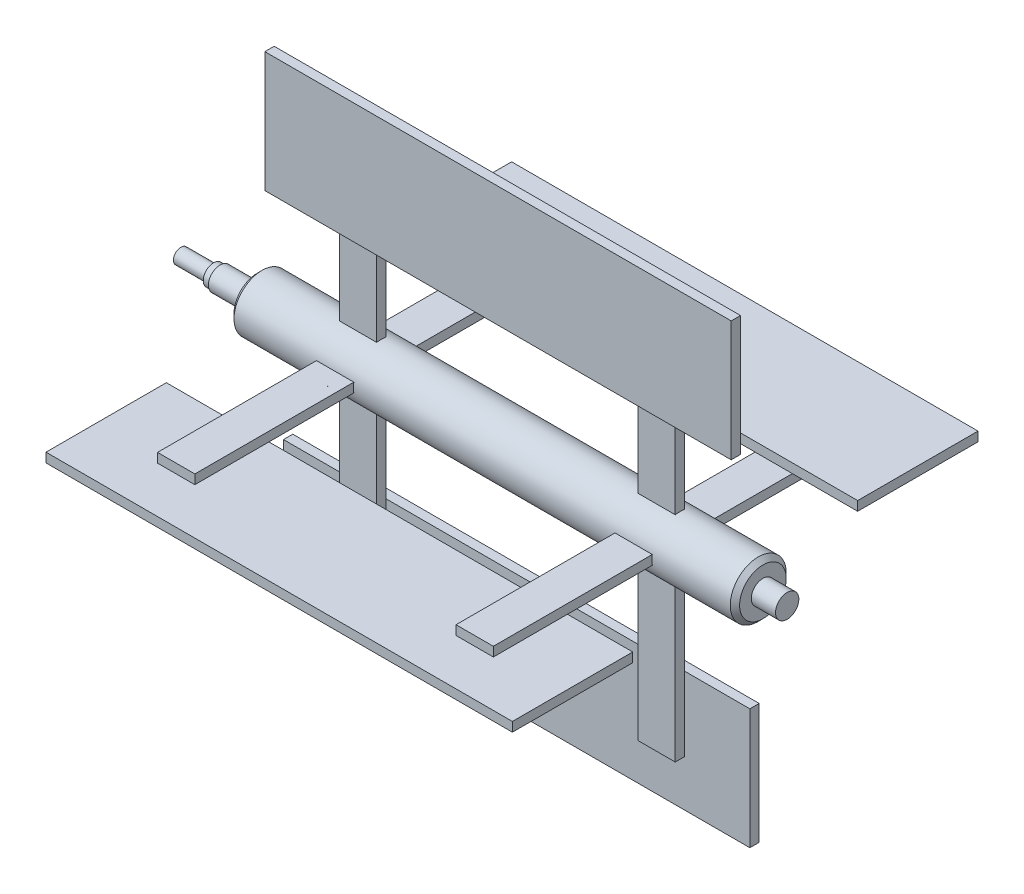
from build123d import *

# Parameters (mm, degrees)
CHAMFER1_SIZE       = 5
SKETCH3_W           = 40
SKETCH3_H           = 200
BOSS_EXTRUDE1_DEPTH = 5
SKETCH4_W           = 500
SKETCH4_H           = 129
BOSS_EXTRUDE2_DEPTH = 10
CIRPATTERN2_COUNT   = 4


with BuildPart() as part:
    # Sketch2 → Revolve1 (revolve)
    with BuildSketch(Plane(origin=(0, 0, 0), x_dir=(1, 0, 0), z_dir=(0, 1, 0))):
        Polygon((-55.931623932, 0), (-55.931623932, 8), (-20.931623932, 8), (-20.931623932, 11), (-13.931623932, 11), (-13.931623932, 12.5), (26.068376068, 12.5), (26.068376068, 30), (568.068376068, 30), (568.068376068, 12.5), (594.068376068, 12.5), (594.068376068, 0), align=None)
    revolve(axis=Axis((0, 0, 0), (-1, 0, 0)))

    # Chamfer1
    chamfer1_edges = [part.edges().sort_by_distance(p)[0] for p in [
        (26.068376068, 0, 30),
        (568.068376068, 0, 30),
    ]]
    chamfer(chamfer1_edges, length=CHAMFER1_SIZE)

    # Sketch3 → Boss-Extrude1 (add, symmetric)
    with BuildSketch(Plane.XY):
        with Locations((139.068376068, 100)):
            Rectangle(SKETCH3_W, SKETCH3_H)
        with Locations((459.068376068, 100)):
            Rectangle(SKETCH3_W, SKETCH3_H)
    boss_extrude1 = extrude(amount=BOSS_EXTRUDE1_DEPTH, both=True)

    # Sketch4 → Boss-Extrude2 (add)
    with BuildSketch(Plane.XY.offset(5)):
        with Locations((299.068376068, 185.080398915)):
            Rectangle(SKETCH4_W, SKETCH4_H)
    boss_extrude2 = extrude(amount=BOSS_EXTRUDE2_DEPTH)

    # CirPattern2: Boss-Extrude1, Boss-Extrude2 ×4 about axis
    cirpattern2_axis = Axis((0, 0, 0), (1, 0, 0))
    add([boss_extrude1.rotate(cirpattern2_axis, i * 360 / CIRPATTERN2_COUNT) for i in range(1, CIRPATTERN2_COUNT)])
    add([boss_extrude2.rotate(cirpattern2_axis, i * 360 / CIRPATTERN2_COUNT) for i in range(1, CIRPATTERN2_COUNT)])


solid = part.part
